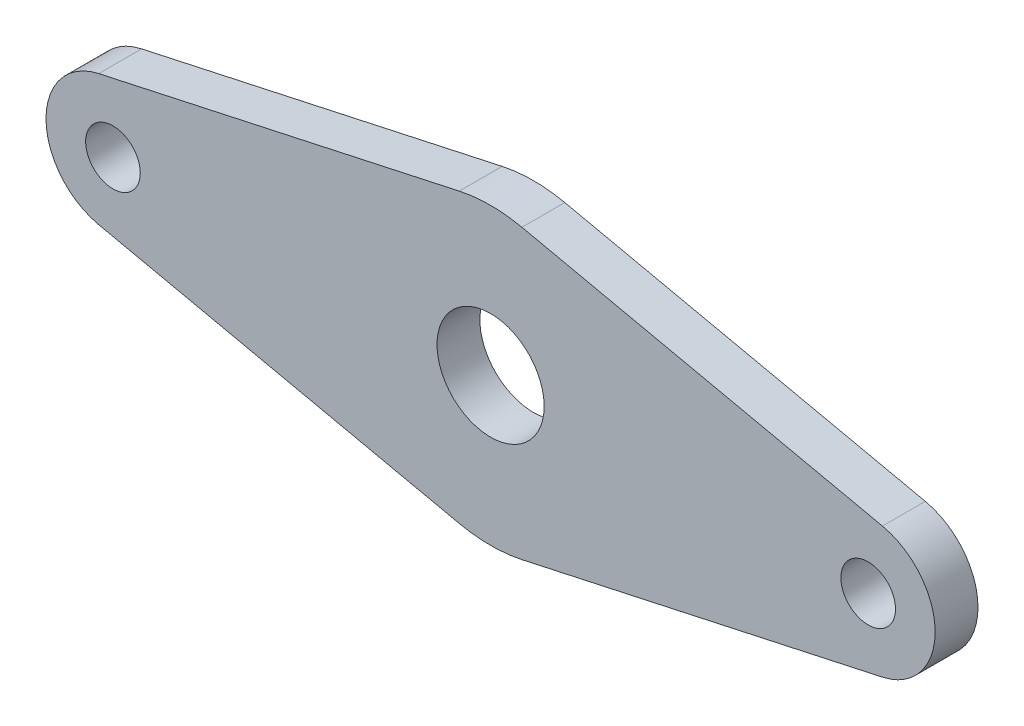
SolidWorks part; units mm, degrees
material "1023 碳钢板 (SS)"
ref_plane "前视基准面" through (0, 0, 0) normal (0, 0, 1) x (1, 0, 0)
ref_plane "上视基准面" through (0, 0, 0) normal (0, 1, 0) x (1, 0, 0)
ref_plane "右视基准面" through (0, 0, 0) normal (1, 0, 0) x (0, 0, -1)
sketch "草图1" plane through (0, 0, 0) normal (0, 0, 1) x (1, 0, 0)
  line L0 (-73.1596, 12.2138) -> (-5.8511, 26.8703)
  line L1 (-73.1596, -12.2138) -> (-5.8511, -26.8703)
  line L2 (5.8511, 26.8703) -> (73.1596, 12.2138)
  line L3 (5.8511, -26.8703) -> (73.1596, -12.2138)
  arc A0 (-5.8511, -26.8703) -> (5.8511, -26.8703) centre (0, 0) ccw
  arc A1 (-73.1596, 12.2138) -> (-73.1596, -12.2138) centre (-70.5, 0) ccw
  arc A2 (73.1596, -12.2138) -> (73.1596, 12.2138) centre (70.5, 0) ccw
  arc A3 (5.8511, 26.8703) -> (-5.8511, 26.8703) centre (0, 0) ccw
  dimension "D1" = 55
  dimension "D4" = 25
  dimension "D5" = 25
  dimension "D2" = 141
  dimension "D3" = 70.5
extrude "凸台-拉伸1" add sketch "草图1" along normal blind 8 contours A2 L2 A3 L0 A1 L1 A0 L3
sketch "草图2" plane through (0, 0, 8) normal (0, 0, 1) x (1, 0, 0)
  circle A0 centre (-70.5, 0) radius 7.429
  circle A1 centre (70.5, 0) radius 4.4823
  dimension "D1" = 141
  dimension "D2" = 70.5
hole_wizard "M12 螺纹孔1" positions "草图3" profile "草图4" tap size "M12" standard "GB"
sketch "草图3" plane through (0, 0, 8) normal (0, 0, 1) x (1, 0, 0)
  point P0 (-70.5, 0)
  point P3 (70.5, 0)
sketch "草图4" plane through (-70.5, 0, 8) normal (1, 0, 0) x (0, -1, 0)
  line L0 (0, 0) -> (0, 32.3144)
  line L1 (0, 32.3144) -> (5.1, 29.25)
  line L2 (5.1, 29.25) -> (5.1, 0)
  line L5 (5.1, 0) -> (0, 0)
  line L10 (0, 32.3144) -> (-5.1, 29.25) construction
  line L11 (0, -6.35) -> (0, 107.95) construction
  dimension "螺纹孔钻头直径" = 10.2
  dimension "螺纹孔钻头深度" = 29.25
  dimension "导头角度" = 118
cosmetic thread "孔螺蚊线1" parameters "D1"=24, "D2"=12
cosmetic thread "孔螺蚊线2" parameters "D1"=24, "D2"=12
sketch "草图5" plane through (0, 0, 8) normal (0, 0, 1) x (1, 0, 0)
  circle A0 centre (0, 0) radius 10
  dimension "D1" = 20
extrude "切除-拉伸1" cut sketch "草图5" against normal blind 8
